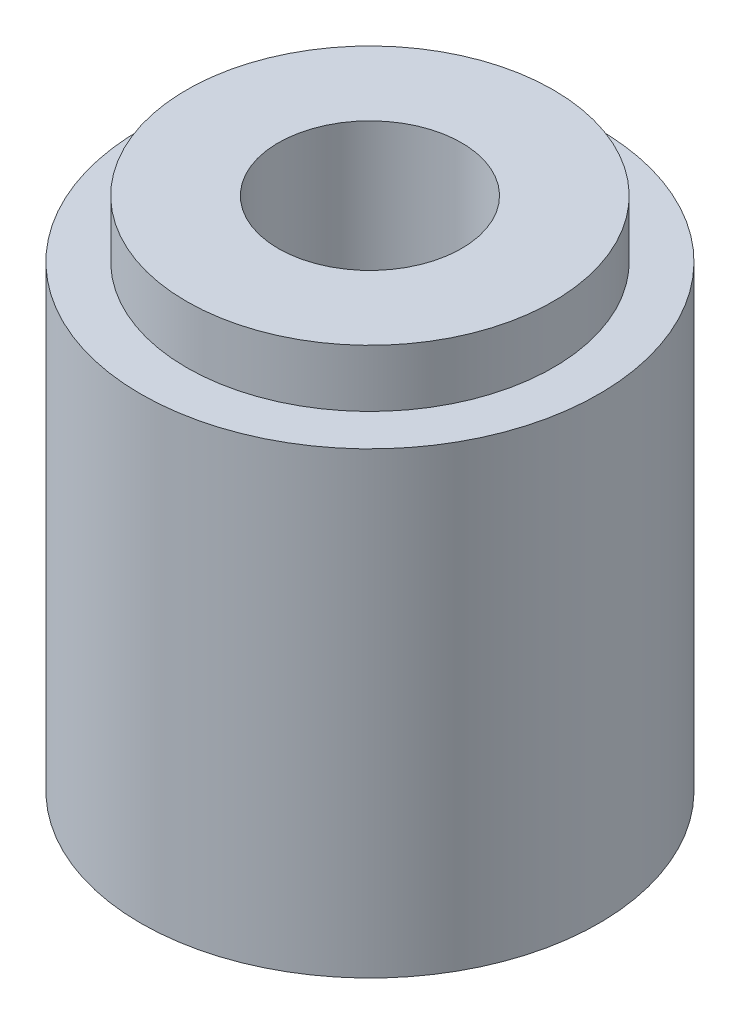
from build123d import *

# Parameters (mm, degrees)
CHAMFER1_SIZE = 3


with BuildPart() as part:
    # Sketch1 → Revolve1 (revolve)
    with BuildSketch(Plane.XY, mode=Mode.PRIVATE) as revolve1_sk:
        Polygon((10.25, 0), (20, 0), (20, 40), (16, 40), (16, 45), (8, 45), (8, 31.299038106), (10.25, 30), align=None)
    revolve(revolve1_sk.sketch.rotate(Axis((0, 45, 0), (0, -1, 0)), 90), axis=Axis((0, 45, 0), (0, -1, 0)))

    # Chamfer1
    chamfer1_edges = [part.edges().sort_by_distance(p)[0] for p in [
        (0, 0, -10.25),
    ]]
    chamfer(chamfer1_edges, length=CHAMFER1_SIZE)


solid = part.part
